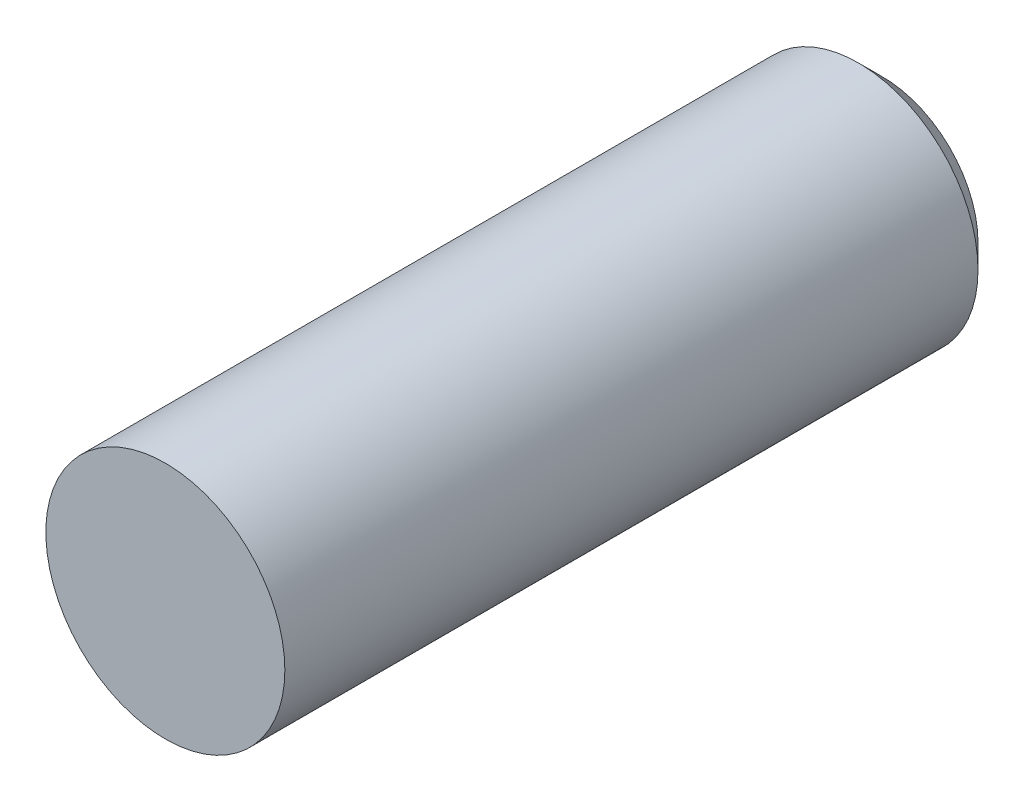
SolidWorks part; units mm, degrees
ref_plane "Front Plane" through (0, 0, 0) normal (0, 0, 1) x (1, 0, 0)
ref_plane "Top Plane" through (0, 0, 0) normal (0, 1, 0) x (1, 0, 0)
ref_plane "Right Plane" through (0, 0, 0) normal (1, 0, 0) x (0, 0, -1)
sketch "Sketch1" plane through (0, 0, 0) normal (0, 0, 1) x (1, 0, 0)
  circle A0 centre (0, 0) radius 5
extrude "Boss-Extrude1" add sketch "Sketch1" along normal blind 30
chamfer "Chamfer1" distance 1 angle 45 1 edges at (5, 0, 0)
